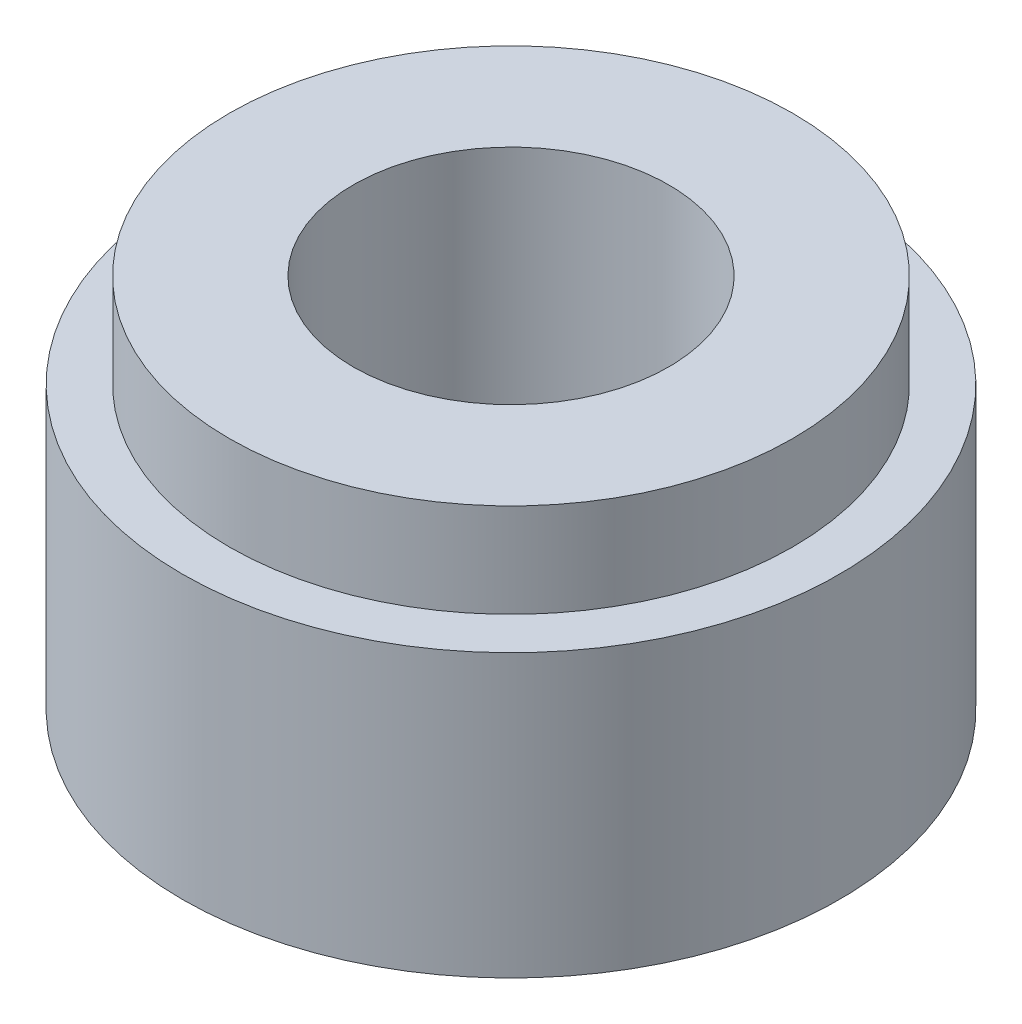
SolidWorks part; units mm, degrees
ref_plane "Front Plane" through (0, 0, 0) normal (0, 0, 1) x (1, 0, 0)
ref_plane "Top Plane" through (0, 0, 0) normal (0, 1, 0) x (1, 0, 0)
ref_plane "Right Plane" through (0, 0, 0) normal (1, 0, 0) x (0, 0, -1)
sketch "Sketch1" plane through (0, 0, 0) normal (0, 1, 0) x (1, 0, 0)
  circle A0 centre (0, 0) radius 17.5
  dimension "D1" = 35
extrude "Boss-Extrude1" add sketch "Sketch1" along normal blind 15
sketch "Sketch2" plane through (0, 15, 0) normal (0, 1, 0) x (1, 0, 0)
  circle A0 centre (0, 0) radius 15
  dimension "D1" = 30
extrude "Boss-Extrude2" add sketch "Sketch2" along normal blind 5
sketch "Sketch3" plane through (0, 20, 0) normal (0, 1, 0) x (1, 0, 0)
  circle A0 centre (0, 0) radius 8.4
  dimension "D1" = 16.8
extrude "Cut-Extrude1" cut sketch "Sketch3" against normal through all
